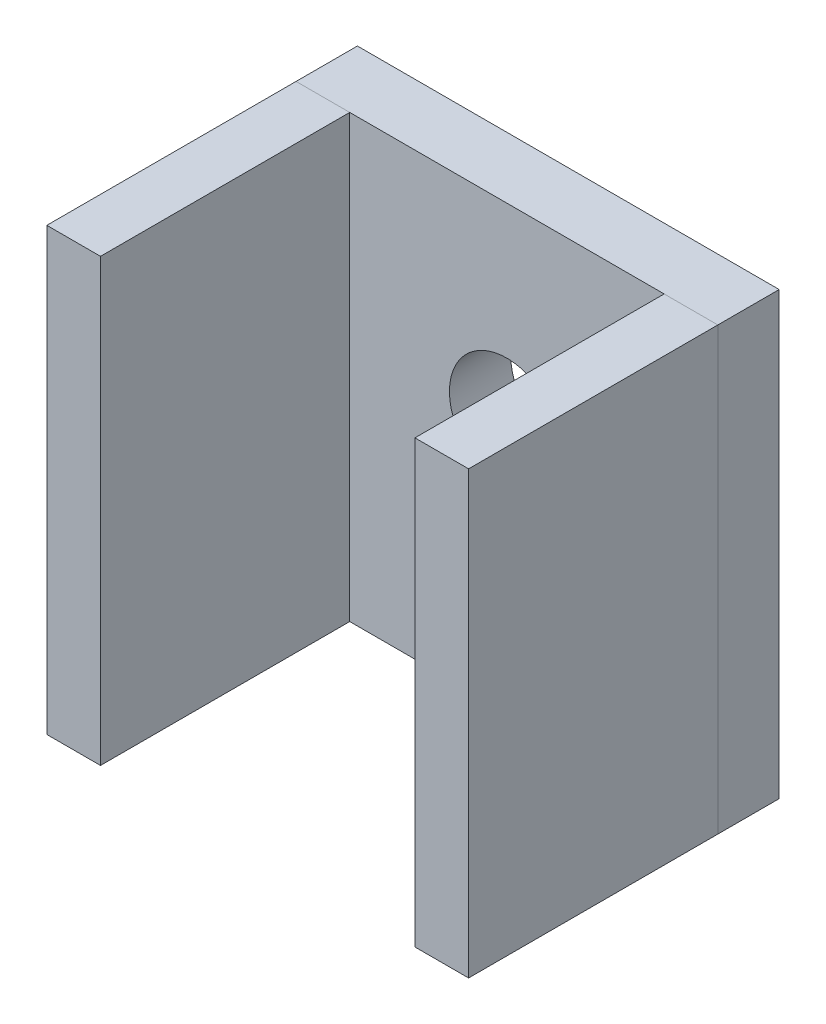
from build123d import *

# Parameters (mm, degrees)
SKETCH_1_W          = 110
SKETCH_1_H          = 100
EXTRUDE_1_DEPTH     = 16
SKETCH_2_W          = 65
SKETCH_2_H          = 115
EXTRUDE_2_DEPTH     = 14
SKETCH_3_R          = 15
CUT_EXTRUDE_1_DEPTH = 16
SKETCH_4_W          = 110
SKETCH_4_H          = 16
EXTRUDE_3_DEPTH     = 15


with BuildPart() as part:
    # 草图1 → 凸台-拉伸1 (new body)
    with BuildSketch(Plane.XY):
        Rectangle(SKETCH_1_W, SKETCH_1_H)
    extrude(amount=EXTRUDE_1_DEPTH)

    # 草图3 → 切除-拉伸1 (cut)
    with BuildSketch(Plane(origin=(0, 0, 0), x_dir=(-1, 0, 0), z_dir=(0, 0, -1))):
        Circle(SKETCH_3_R)
    extrude(amount=-CUT_EXTRUDE_1_DEPTH, mode=Mode.SUBTRACT)

    # 草图4 → 凸台-拉伸3 (add)
    with BuildSketch(Plane.XZ.offset(50)):
        with Locations((0, 8)):
            Rectangle(SKETCH_4_W, SKETCH_4_H)
    extrude(amount=EXTRUDE_3_DEPTH)


with BuildPart() as body_2:
    # 草图2 → 凸台-拉伸2 (new body)
    with BuildSketch(Plane.ZY.offset(55)):
        with Locations((48.5, -7.5)):
            Rectangle(SKETCH_2_W, SKETCH_2_H)
    extrude(amount=-EXTRUDE_2_DEPTH)


with BuildPart() as body_3:
    # 镜向1: mirrored copy
    add(body_2.part.mirror(Plane(origin=(0, 0, 0), x_dir=(0, 0, 1), z_dir=(1, 0, 0))))


solid = Compound([part.part, body_2.part, body_3.part])
